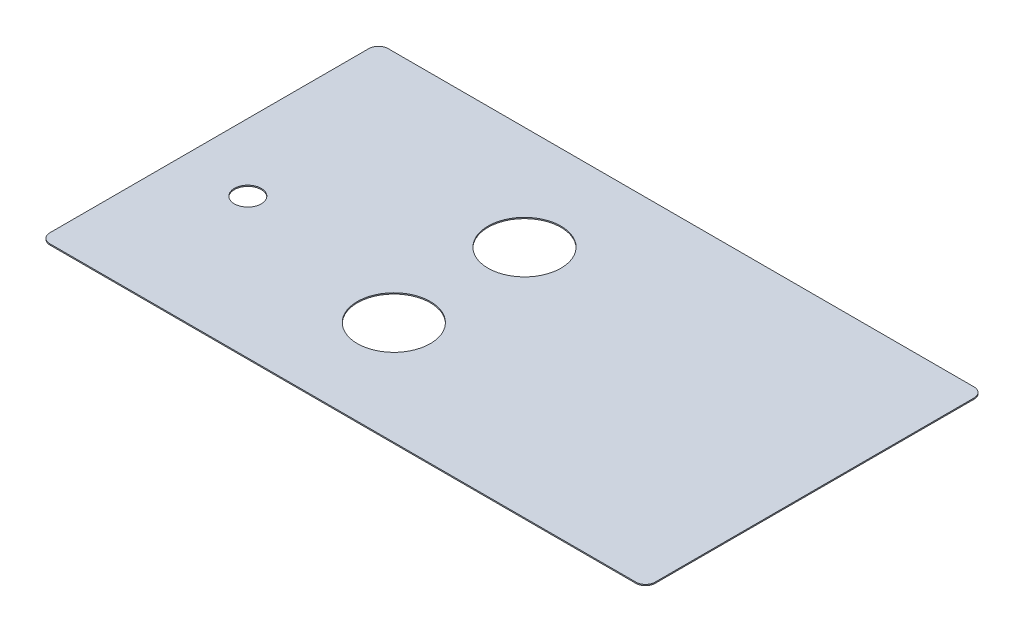
SolidWorks part; units mm, degrees
material "35"
ref_plane "Front Plane" through (0, 0, 0) normal (0, 0, 1) x (1, 0, 0)
ref_plane "Top Plane" through (0, 0, 0) normal (0, 1, 0) x (1, 0, 0)
ref_plane "Right Plane" through (0, 0, 0) normal (1, 0, 0) x (0, 0, -1)
sketch "Sketch1" plane through (0, 0, 0) normal (0, 1, 0) x (1, 0, 0)
  line L0 (-215.8997, 0) -> (34.3319, 0) construction
  line L1 (0, 95.2615) -> (0, -113.2991) construction
  line L2 (-130, 83) -> (-130, -83)
  line L3 (-125, 88) -> (180, 88)
  line L5 (-125, -88) -> (180, -88)
  line L6 (185, 83) -> (185, -83)
  arc A0 (180, -88) -> (185, -83) centre (180, -83) ccw
  arc A1 (185, 83) -> (180, 88) centre (180, 83) ccw
  arc A2 (-125, -88) -> (-130, -83) centre (-125, -83) cw
  arc A3 (-125, 88) -> (-130, 83) centre (-125, 83) ccw
  circle A7 centre (0, 34) radius 19
  circle A8 centre (0, -34) radius 19
  circle A9 centre (-95, -15) radius 7
  dimension "D6" = 5
  dimension "D10" = 38
  dimension "D11" = 14
  dimension "D2" = 176
  dimension "D4" = 130
  dimension "D5" = 315
  dimension "D7" = 15
  dimension "D8" = 95
  dimension "D9" = 68
extrude "Boss-Extrude1" add sketch "Sketch1" along normal mid plane 0.6
